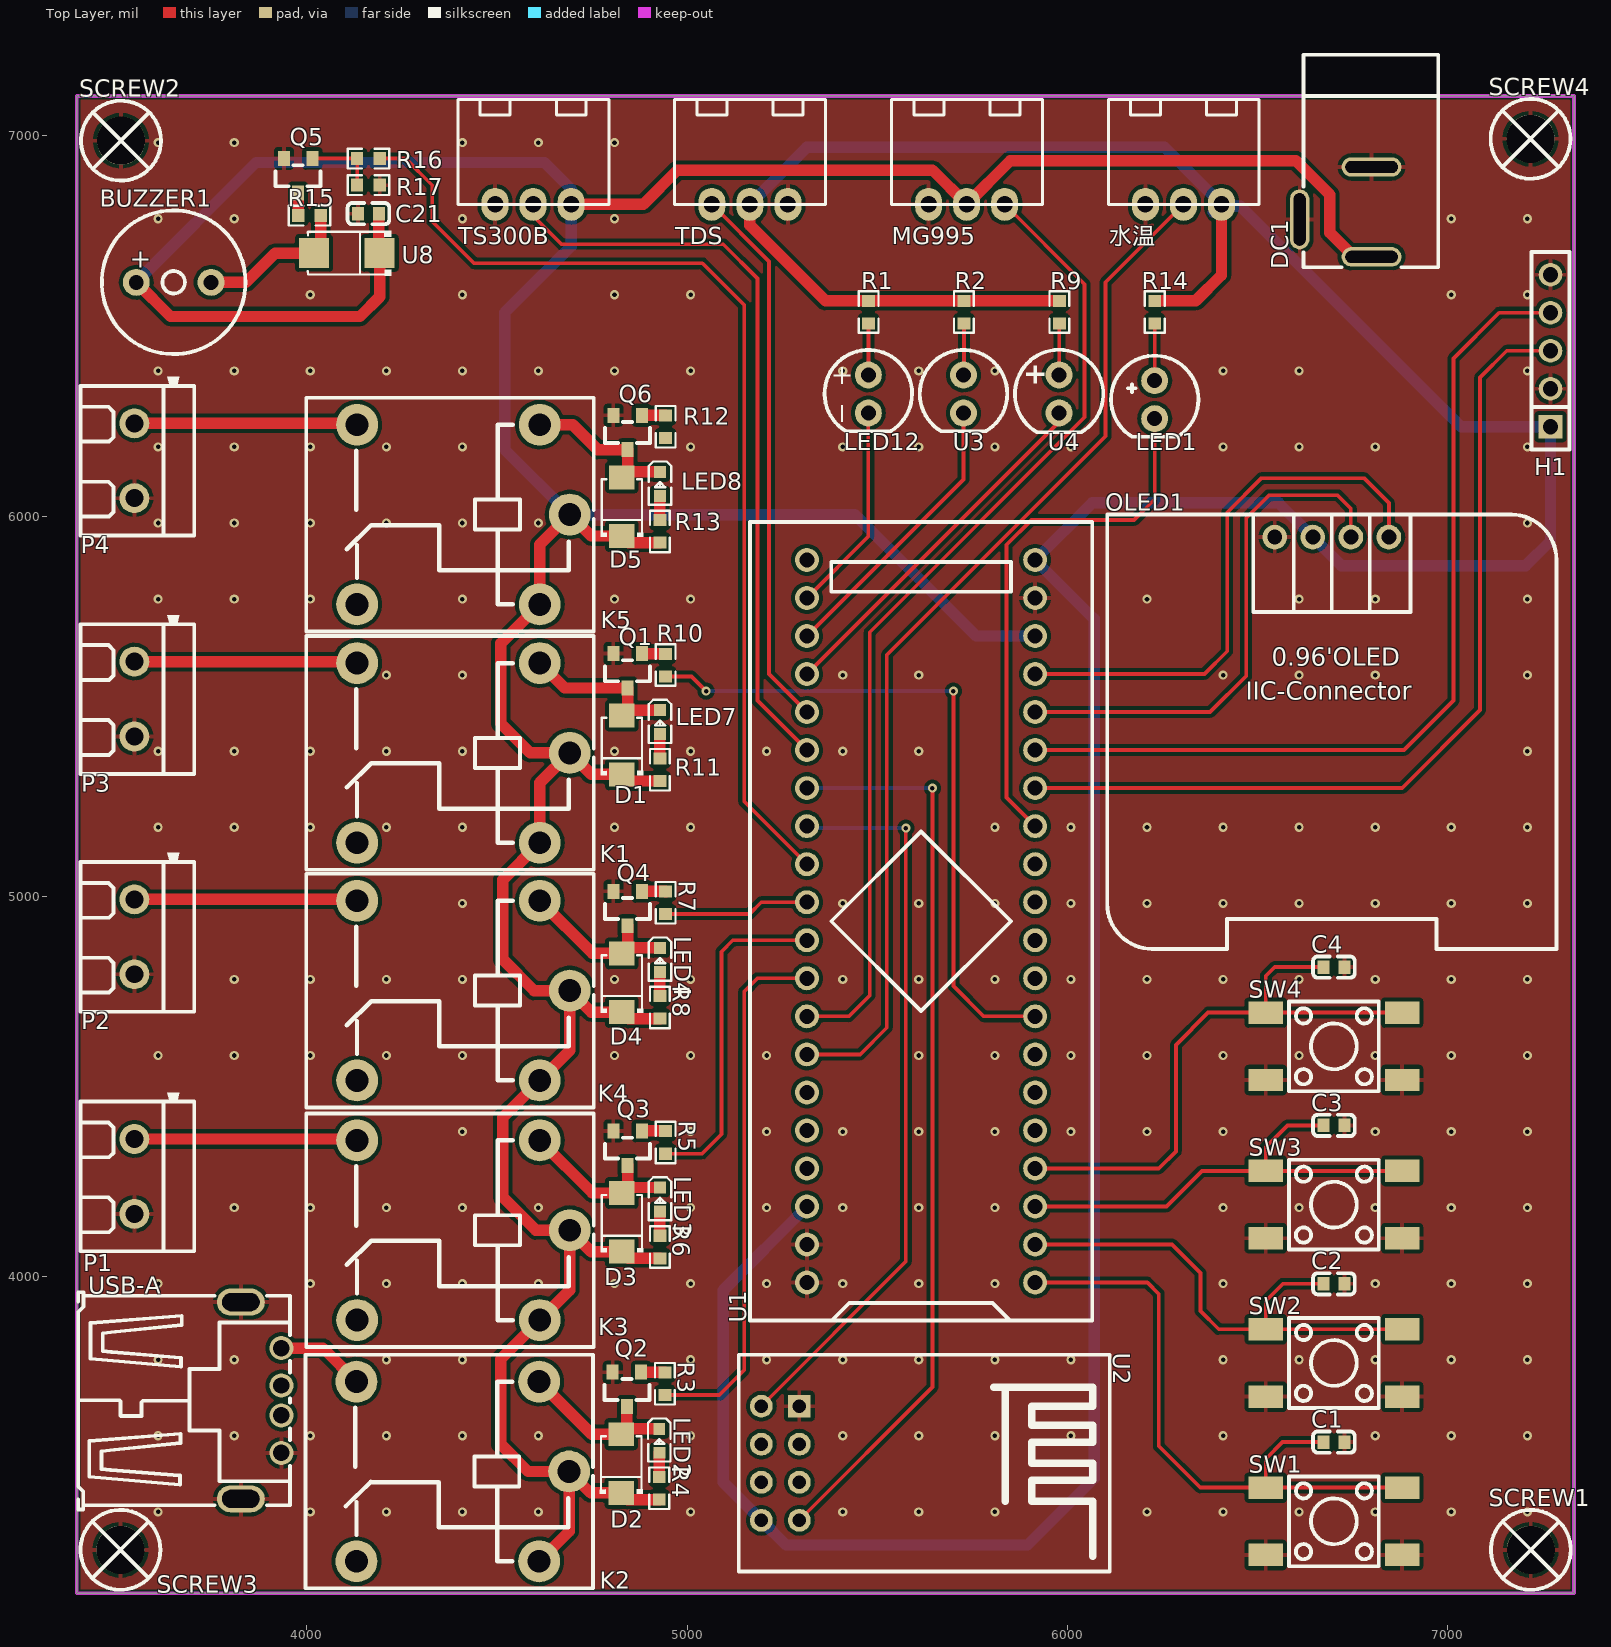
[diagram p0: Top Layer view]
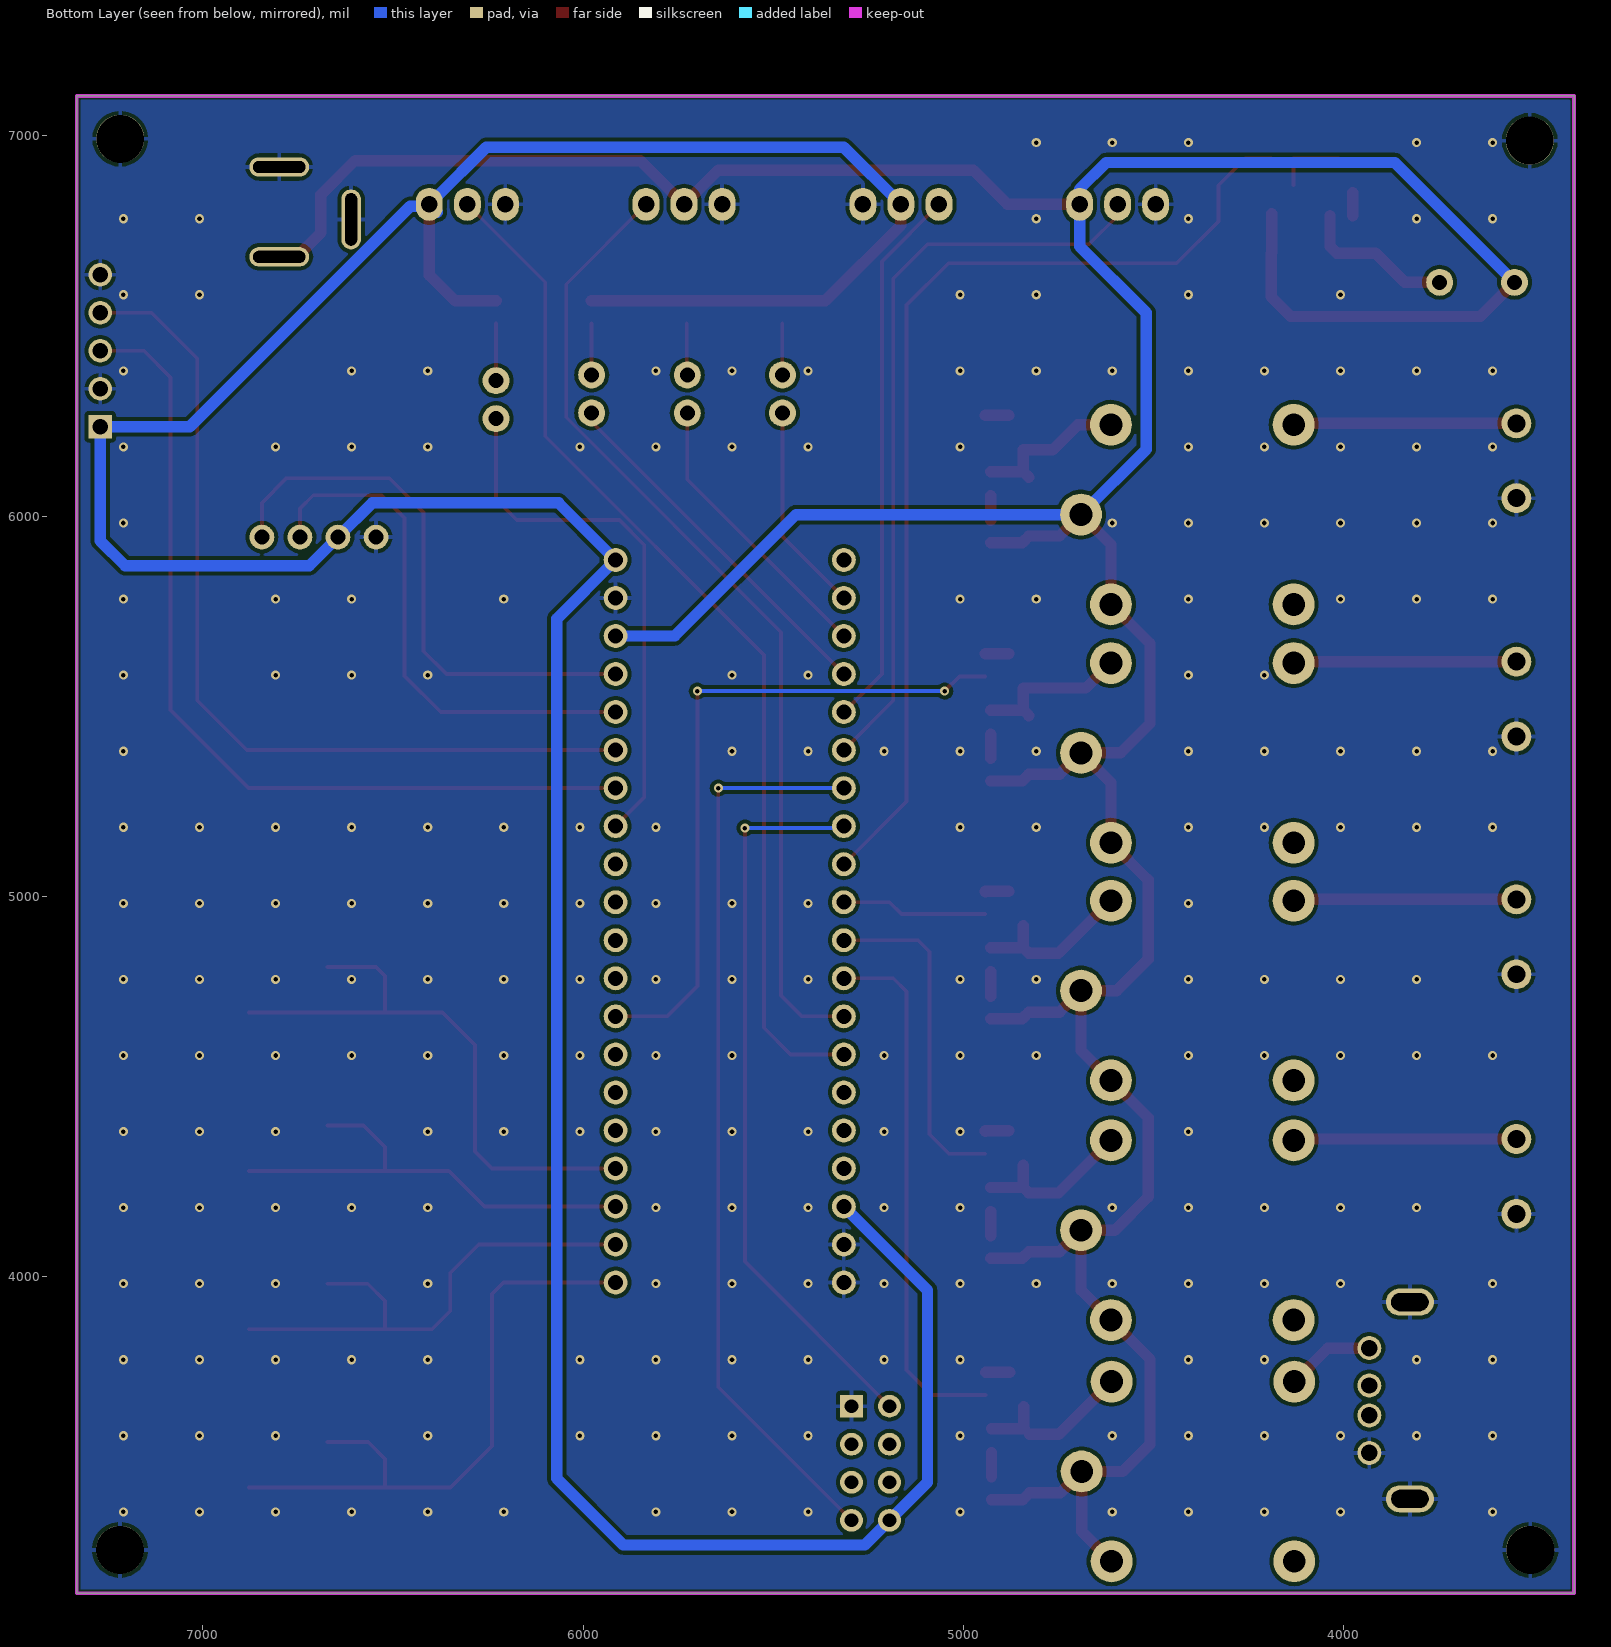
[diagram p1: Bottom Layer view, seen from below]
# Altium PCB MISC51727.pcbdoc
Units mil, origin at the board's own origin, x right, y up, seen from the top; angles counter-clockwise.
Board outline 3937.01 x 3937.01 mil, 2 copper layers (Top Layer, Bottom Layer), stack 62.206 mil thick; 71 components, 56 nets, 225 pads, 231 vias.

## Layer stack, top to bottom
Top Solder Mask Layer: solder mask 0.394, Dk 3.3
Top Layer: signal copper 1.379
Dielectric1: surface 59.449, FR4, Dk 4.5
Bottom Layer: signal copper 1.378
Bottom Solder Mask Layer: solder mask 0.394, Dk 3.3

## Board outline
3395,7105 3395,3167.99 7332.01,3167.99 7332.01,7105

## Design rules (kind name [scope] priority, off if disabled: settings)
BoardOutlineClearance copperThickness2oz_1 [All] p2 off: genericclearance=7.99 ignorepadtopadclearanceinfootprint=FALSE except(0: Arc-SplitContinuation Track-SplitContinuation SMDPad-SplitContinuation THPad-SplitContinuation Via-SplitContinuation Fill-SplitContinuation Region-SplitContinuation Poly-SplitContinuation Text-SplitContinuation Hole-SplitContinuation; 5.98: Arc-CutoutEdge SMDPad-CutoutEdge THPad-CutoutEdge Via-CutoutEdge Fill-CutoutEdge Region-CutoutEdge Text-CutoutEdge; 6.93: Hole-OutlineEdge Hole-CutoutEdge; 10: Poly-OutlineEdge Poly-CutoutEdge; 11.81: Arc-OutlineEdge Track-OutlineEdge SMDPad-OutlineEdge THPad-OutlineEdge Via-OutlineEdge Fill-OutlineEdge Region-OutlineEdge Text-OutlineEdge Track-CutoutEdge)
BoardOutlineClearance copperThickness1oz_1 [All] p4: genericclearance=4.02 ignorepadtopadclearanceinfootprint=FALSE except(0: Arc-SplitContinuation Track-SplitContinuation SMDPad-SplitContinuation THPad-SplitContinuation Via-SplitContinuation Fill-SplitContinuation Region-SplitContinuation Poly-SplitContinuation Text-SplitContinuation Hole-SplitContinuation; 6: SMDPad-CutoutEdge THPad-CutoutEdge Via-CutoutEdge Fill-CutoutEdge Region-CutoutEdge Text-CutoutEdge; 6.93: Hole-OutlineEdge Hole-CutoutEdge; 10: Poly-OutlineEdge Poly-CutoutEdge; 11.8: Arc-OutlineEdge Track-OutlineEdge SMDPad-OutlineEdge THPad-OutlineEdge Via-OutlineEdge Fill-OutlineEdge Region-OutlineEdge Text-OutlineEdge; 11.81: Arc-CutoutEdge Track-CutoutEdge)
Clearance copperThickness2oz [All] p1 off: gap=7.99 ignorepadtopadclearanceinfootprint=FALSE except(5.98: SMDPad-Track SMDPad-SMDPad THPad-Track SMDPad-THPad THPad-THPad Track-Via SMDPad-Via THPad-Via Via-Via Fill-Track Region-Track Fill-SMDPad Region-SMDPad Fill-THPad Region-THPad Fill-Via Region-Via Fill-Fill Fill-Region Region-Region Arc-Track Arc-SMDPad Arc-THPad Arc-Via Fill-Arc Region-Arc Arc-Arc Text-Track SMDPad-Text Text-THPad Text-Via Fill-Text Region-Text Arc-Text Text-Text; 6.93: Hole-Track Hole-SMDPad Hole-THPad Hole-Via Fill-Hole Region-Hole Hole-Arc Hole-Text; 10: Poly-Track Poly-SMDPad Poly-THPad Poly-Via Poly-Fill Poly-Region Poly-Poly Poly-Arc Poly-Text Poly-Hole)
Clearance copperThickness1oz [All] p3: gap=4.02 ignorepadtopadclearanceinfootprint=FALSE except(5.98: SMDPad-Track SMDPad-SMDPad THPad-Track SMDPad-THPad THPad-THPad Track-Via SMDPad-Via THPad-Via Via-Via Fill-Track Region-Track Fill-SMDPad Region-SMDPad Fill-THPad Region-THPad Fill-Via Region-Via Fill-Fill Fill-Region Region-Region; 6: Arc-Track Arc-SMDPad Arc-THPad Arc-Via Fill-Arc Region-Arc Arc-Arc Text-Track SMDPad-Text Text-THPad Text-Via Fill-Text Region-Text Arc-Text Text-Text; 6.93: Hole-Track Hole-SMDPad Hole-THPad Hole-Via Fill-Hole Region-Hole Hole-Arc Hole-Text; 10: Poly-Track Poly-SMDPad Poly-THPad Poly-Via Poly-Fill Poly-Region Poly-Poly Poly-Arc Poly-Text Poly-Hole)
Creepage creepage [All] p1: checkdistance=0 ignoreinternallayers=TRUE applytopolygonpour=TRUE
DiffPairsRouting differentialPair [All] p1: maxlimit=6 minlimit=6 mostfreqgap=6 toplayer_minwidth=5 toplayer_prefwidth=10 toplayer_maxwidth=100 toplayer_mingap=6 toplayer_prefgap=6 toplayer_maxgap=6 bottomlayer_minwidth=5 bottomlayer_prefwidth=10 bottomlayer_maxwidth=100 bottomlayer_mingap=6 bottomlayer_prefgap=6 bottomlayer_maxgap=6 maxuncoupledlength=10
HoleToHoleClearance otherClearance [All] p1: gap=11.81 allowstackedmicrovias=TRUE
Length netLength [All] p1: minlimit=0 maxlimit=0
MatchedLengths netLengthTolerance [All] p1: tolerance=1000
PasteMaskExpansion pasteMaskExpansion [All] p1: expansion=0
PlaneConnect innerPlane [All] p1: planeconnectstyle=Relief reliefexpansion=20 reliefentries=4 reliefconductorwidth=10 reliefairgap=10
PolygonConnect copperRegion [(InNet('GND'))] p1: connectstyle=Relief reliefconductorwidth=10 reliefentries=4 polygonreliefangle="90 Angle" airgapwidth=10 via.connectstyle=Relief via.reliefconductorwidth=10 via.reliefentries=4 via.polygonreliefangle="90 Angle" via.airgapwidth=10
RoutingVias viaSize [All] p1: holewidth=12.01 width=24.02 viastyle="Through Hole" minholewidth=11.81 minwidth=19.68 maxholewidth=248.03 maxwidth=393.7
SolderMaskExpansion solderMaskExpansion [IsVia] p1: expansion=-1000 istentingtop=TRUE
SolderMaskExpansion solderMaskExpansion [All] p2: expansion=2 istentingtop=FALSE
Width copperThickness2oz_2 [All] p1 off: maxlimit=100 minlimit=8 preferedwidth=10
Width copperThickness1oz_2 [All] p2: maxlimit=100 minlimit=5 preferedwidth=10

## Components (designator, comment, footprint, x,y, rotation, side; value= is the part's Value field where it differs from the comment)
BUZZER1 "3kHz" BUZ-TH_BD9.6-P5.00-D0.7-FD 3650,6615 r0 top
C1 "100nF" C0603 6700.55,3565.55 r0 top
C2 "100nF" C0603 6700.55,3981.81 r0 top
C3 "100nF" C0603 6700.55,4398.07 r0 top
C4 "100nF" C0603 6700.55,4814.33 r0 top
C21 "100nF" C0603 4162.11,6795.28 r0 top
D1 "M7F" SMAF_L3.5-W2.6-LS4.7-RD 4828.38,5398.43 r90 top
D2 "M7F" SMAF_L3.5-W2.6-LS4.7-RD 4826.72,3509.06 r90 top
D3 "M7F" SMAF_L3.5-W2.6-LS4.7-RD 4828.38,4143.43 r90 top
D4 "M7F" SMAF_L3.5-W2.6-LS4.7-RD 4828.38,4773.43 r90 top
D5 "M7F" SMAF_L3.5-W2.6-LS4.7-RD 4828.38,6025.08 r90 top
DC1 "" DC-2.0 6810,6805 r90 top
H1 "" HDR-TH_5P-P2.54-V-F 7270,6435 r90 top
K1 "SRD-DC5V-SL-C" RELAY-TH_SRD-DCXXV-SL-C 4411.82,5377.66 r180 top
K2 "SRD-DC5V-SL-C" RELAY-TH_SRD-DCXXV-SL-C 4410.16,3488.29 r180 top
K3 "SRD-DC5V-SL-C" RELAY-TH_SRD-DCXXV-SL-C 4411.82,4122.66 r180 top
K4 "SRD-DC5V-SL-C" RELAY-TH_SRD-DCXXV-SL-C 4411.82,4752.66 r180 top
K5 "SRD-DC5V-SL-C" RELAY-TH_SRD-DCXXV-SL-C 4411.82,6004.31 r180 top
LED1 "blue" LED-TH_BD5.9-P2.54-RD_BLUE 6229.4,6306.44 r90 top
LED2 "MS-PTV1608NWAF-B02" LED0603-RD 4926.72,3569.06 r270 top
LED3 "MS-PTV1608NWAF-B02" LED0603-RD 4928.38,4203.43 r270 top
LED4 "MS-PTV1608NWAF-B02" LED0603-RD 4928.38,4833.43 r270 top
LED7 "MS-PTV1608NWAF-B02" LED0603-RD 4928.38,5458.43 r270 top
LED8 "MS-PTV1608NWAF-B02" LED0603-RD 4928.38,6085.08 r270 top
LED12 "red" LED-TH_BD5.9-P2.54-RD_RED 5476.39,6321.24 r90 top
MG995 "" XH2.54-3P 5735,6820 r0 top
OLED1 "" 0.96OLED_4P 6695,5945 r0 top
P1 "KF301-2P terminal block" CONN-TH_XY301V-A-5.0-2P 3546.72,4264.06 r90 top
P2 "KF301-2P terminal block" CONN-TH_XY301V-A-5.0-2P 3546.72,4894.06 r90 top
P3 "KF301-2P terminal block" CONN-TH_XY301V-A-5.0-2P 3546.72,5519.06 r90 top
P4 "KF301-2P terminal block" CONN-TH_XY301V-A-5.0-2P 3546.72,6145.71 r90 top
Q1 "" S8050_SOT-23 4848.38,5593.43 r90 top
Q2 "" S8050_SOT-23 4846.72,3704.06 r90 top
Q3 "" S8050_SOT-23 4848.38,4338.43 r90 top
Q4 "" S8050_SOT-23 4848.38,4968.43 r90 top
Q5 "" S8050_SOT-23 3982.11,6895.28 r90 top
Q6 "" S8050_SOT-23 4848.38,6220.08 r90 top
R1 "1K" R0603 5477.06,6536.64 r270 top
R2 "1K" R0603 5727.84,6536.64 r270 top
R3 "330" R0603 4941.72,3719.06 r270 top
R4 "1K" R0603 4926.72,3444.06 r270 top
R5 "330" R0603 4943.38,4353.43 r270 top
R6 "1K" R0603 4928.38,4078.43 r270 top
R7 "330" R0603 4943.38,4983.43 r270 top
R8 "1K" R0603 4928.38,4708.43 r270 top
R9 "1K" R0603 5978.62,6536.64 r270 top
R10 "330" R0603 4943.38,5608.43 r270 top
R11 "1K" R0603 4928.38,5333.43 r270 top
R12 "330" R0603 4943.38,6235.08 r270 top
R13 "1K" R0603 4928.38,5960.08 r270 top
R14 "1K" R0603 6229.4,6536.64 r270 top
R15 "0R" R0603 4007.11,6790.28 r0 top
R16 "1K" R0603 4162.11,6940.28 r0 top
R17 "4.7K" R0603 4162.11,6870.28 r0 top
SCREW1 "" M3螺丝 7218.26,3282.26 r0 top
SCREW2 "" M3螺丝 3511.56,6987.26 r0 top
SCREW3 "" M3螺丝 3510,3282.26 r0 top
SCREW4 "" M3螺丝 7217.52,6992.26 r0 top
SW1 "" SW-SMD_4P-L6.0-W6.0-P4.50-LS9.0-2 6700.55,3357.42 r0 top
SW2 "" SW-SMD_4P-L6.0-W6.0-P4.50-LS9.0-2 6700.55,3773.68 r0 top
SW3 "" SW-SMD_4P-L6.0-W6.0-P4.50-LS9.0-2 6700.55,4189.94 r0 top
SW4 "" SW-SMD_4P-L6.0-W6.0-P4.50-LS9.0-2 6700.55,4606.2 r0 top
TDS "" XH2.54-3P 5165,6820 r0 top
TS300B "" XH2.54-3P 4595,6820 r0 top
U1 "LCKFB-DKX-STM32F103C8T6" CONN-TH_L53.3-W22.9_STM32F103C8T6-CARD 5615,4935 r90 top
U2 "ESP8266-01S" WIFIM-TH_ESP8266-01S 5245,3510 r270 top
U3 "green" LED-TH_BD5.9-P2.54-RD_GREEN 5726.63,6321.14 r90 top
U4 "yellow" LED-TH_BD5.9-P2.54-RD_YELLOW 5977.95,6321.4 r90 top
U8 "SS24-MS" SMA_L4.3-W2.6-LS5.1-RD 4105.13,6691.58 r180 top
USB-A "USB-AF" USB-A-TH_USB-302-T 3880,3675 r270 top
水温 "" XH2.54-3P 6305,6820 r0 top

## Footprints (in the part's own frame and the unit in brackets; to place one, negate y for a bottom-side part, rotate by r counter-clockwise, add the part's x,y. Pads: shape width x height; smd on the part's side, far side on the other; paste and mask are expansions set on the pad)
0.96OLED_4P [mm]
  round 1.65 hole 1 copper offset 0,0: 1(-3.81,-0.001) 2(-1.27,0.002) 3(1.27,0.002) 4(3.81,0.002)
  silkscreen extent -15,-27.5 15,1.5
BUZ-TH_BD9.6-P5.00-D0.7-FD [mm]
  round 1.8 hole 1: 1(-2.5,0) 2(2.5,0)
  silkscreen extent -4.8,-4.8 4.8,4.8
C0603 [mm]
  rect 0.8x0.9 smd: 1(-0.7,0) 2(0.7,0)
  silkscreen extent -1.39,-0.71 1.39,0.71
CONN-TH_L53.3-W22.9_STM32F103C8T6-CARD [mm]
  round 1.6 hole 1: 1(-24.13,-7.62) 2(-21.59,-7.62) 3(-19.05,-7.62) 4(-16.51,-7.62) 5(-13.97,-7.62) 6(-11.43,-7.62) 7(-8.89,-7.62) 8(-6.35,-7.62) 9(-3.81,-7.62) 10(-1.27,-7.62) 11(1.27,-7.62) 12(3.81,-7.62) 13(6.35,-7.62) 14(8.89,-7.62) 15(11.43,-7.62) 16(13.97,-7.62) 17(16.51,-7.62) 18(19.05,-7.62) 19(21.59,-7.62) 20(24.13,-7.62) 21(24.13,7.62) 22(21.59,7.62) 23(19.05,7.62) 24(16.51,7.62) 25(13.97,7.62) 26(11.43,7.62) 27(8.89,7.62) 28(6.35,7.62) 29(3.81,7.62) 30(1.27,7.62) 31(-1.27,7.62) 32(-3.81,7.62) 33(-6.35,7.62) 34(-8.89,7.62) 35(-11.43,7.62) 36(-13.97,7.62) 37(-16.51,7.62) 38(-19.05,7.62) 39(-21.59,7.62) 40(-24.13,7.62)
  silkscreen extent -26.67,-11.43 26.67,11.43
CONN-TH_XY301V-A-5.0-2P [mm]
  round 2 hole 1.2: 1(-2.5,0) 2(2.5,0)
  silkscreen extent -5,-4 5.6,3.6
DC-2.0 [mil]
  oval 157.5x51.2 hole 31.5 slot 137.8 at 0 deg paste+0 mask+2: 2(-24.7,199.5)
  oval 51.2x157.5 hole 31.5 slot 137.8 at 90 deg paste+0 mask+2: 3(113.1,10.5) 4(-123.1,10.5)
  silkscreen extent -151,-165 408,190
HDR-TH_5P-P2.54-V-F [mil]
  rect 62x62 hole 40.16: 1(-200,0)
  round 62 hole 40.16: 2(-100,0) 3(0,0) 4(100,0) 5(200,0)
  silkscreen extent -260,-50 260,50
LED0603-RD [mm]
  rect 0.8x0.8 smd: 1(-0.799,0) 2(0.799,0)
  silkscreen extent -1.49,-0.75 1.39,0.76
LED-TH_BD5.9-P2.54-RD_BLUE [mm]
  round 1.8 hole 1 paste+0 mask+0.05: 1(-1.27,0) 2(1.27,0)
  silkscreen extent -2.49,-2.92 2.93,2.92
LED-TH_BD5.9-P2.54-RD_GREEN [mm]
  round 1.8 hole 1 paste+0 mask+0.05: 1(-1.27,0) 2(1.27,0)
  silkscreen extent -2.49,-2.92 2.94,2.92
LED-TH_BD5.9-P2.54-RD_RED [mm]
  round 1.8 hole 1 paste+0 mask+0.05: 1(-1.27,0) 2(1.27,0)
  silkscreen extent -2.49,-2.92 2.94,2.92
LED-TH_BD5.9-P2.54-RD_YELLOW [mm]
  round 1.8 hole 1 paste+0 mask+0.05: 1(-1.27,0) 2(1.27,0)
  silkscreen extent -2.55,-2.95 2.95,2.95
M3螺丝 [mil]
  round 126 hole 126 paste+0 mask+4: 1(0,0)
  silkscreen extent -105,-105 105,105
R0603 [mil]
  rect 31.75x34.02 smd paste-3937.01 mask+2: 1(-29.66,0) 2(29.66,0)
  silkscreen extent -55,-26 55,26
RELAY-TH_SRD-DCXXV-SL-C [mil]
  round 110 hole 60: 1(-200.79,-236.22) 2(279.53,-236.2) 3(279.53,236.2) 4(-200.79,236.22) 5(-279.53,0)
  silkscreen extent -342,-307 413,307
S8050_SOT-23 [mm]
  rect 1x0.8 smd paste+0 mask+0.051: 1(1.15,-0.823) 2(1.15,1.077) 3(-1.15,0.127)
  silkscreen extent -0.7,-1.37 0.7,1.63
SMA_L4.3-W2.6-LS5.1-RD [mm]
  rect 2x2 smd: 1(-2.2,0) 2(2.2,0)
  silkscreen extent -2.98,-1.5 2.6,1.5
SMAF_L3.5-W2.6-LS4.7-RD [mm]
  rect 1.6x1.7 smd: 1(-1.96,0) 2(1.96,0)
  silkscreen extent -2.01,-1.43 1.83,1.42
SW-SMD_4P-L6.0-W6.0-P4.50-LS9.0-2 [mm]
  rect 2.3x1.5 smd: 1(-4.55,2.25) 2(4.55,2.25) 3(-4.55,-2.25) 4(4.55,-2.25)
  silkscreen extent -3,-3 3,3
USB-A-TH_USB-302-T [mm]
  round 1.6 hole 1.1: 1(-3.5,1.355) 2(-1,1.355) 3(1,1.355) 4(3.5,1.355)
  oval 1.8x3.2 hole 1.2 slot 2.5 at 90 deg copper offset -0.001,-0.001: 5(-6.569,-1.354)
  oval 1.8x3.2 hole 1.2 slot 2.5 at 90 deg copper offset 0.001,0.001: 6(6.569,-1.356)
  silkscreen extent -7.23,-12.21 7.28,1.92
WIFIM-TH_ESP8266-01S [mil]
  rect 60x60 hole 36 paste+0 mask+1.97: 1(-150,50)
  round 60 hole 36 paste+0 mask+1.97: 2(-50,50) 3(50,50) 4(150,50) 5(-150,-50) 6(-50,-50) 7(50,-50) 8(150,-50)
  silkscreen extent -285,-109 285,866
XH2.54-3P [mm]
  oval 1.8x2.2 hole 1.1 paste+0 mask+0.102: 1(-2.54,0) 2(0,0) 3(2.54,0)
  silkscreen extent -5.02,0 5.05,7

## Via types
v1: diameter 24.02, hole 12, Top Layer to Bottom Layer, 231 vias

## Nets (pads, with @x,y where several pads share a name; then routed paths per layer and width w, separated by ;. In a path a pad name is that pad's centre, name@x,y a point inside that pad or via, vN(x,y) a via of type N, cw(c..) or ccw(c..) an arc to the next point about the centre after c; other vN are vias at no path point)
$1N2314: Q2.1 R3.1 | length 62.9
  Top Layer w30: Q2.1 4941.11,3749.34 R3.1
$1N2315: D2.2 K2.1 LED2.1 Q2.3 | length 417.3
  Top Layer w30: K2.1 4749.24,3586.23 D2.2 ; Q2.3 4841.72,3601.23 4841.03,3600.54 LED2.1
$1N2316: LED2.2 R4.1 | length 63.9
  Top Layer w30: R4.1 LED2.2
$1N2322: D3.2 K3.1 LED3.1 Q3.3 | length 437.5
  Top Layer w30: K3.1 4750.89,4220.6 D3.2 D3.2@4842.69,4234.91 ; Q3.3 4843.38,4235.6 D3.2@4842.69,4234.91 ; LED3.1 D3.2@4842.69,4234.91
$1N2323: LED3.2 R6.1 | length 63.9
  Top Layer w30: R6.1 LED3.2
$1N2328: Q3.1 R5.1 | length 62.9
  Top Layer w30: Q3.1 4942.76,4383.71 R5.1
$1N2330: Q4.1 R7.1 | length 62.9
  Top Layer w30: Q4.1 4942.76,5013.71 R7.1
$1N2331: D4.2 K4.1 LED4.1 Q4.3 | length 437.5
  Top Layer w30: K4.1 4750.89,4850.6 D4.2 D4.2@4842.69,4864.91 ; Q4.3 4843.38,4865.6 D4.2@4842.69,4864.91 ; LED4.1 D4.2@4842.69,4864.91
$1N2332: LED4.2 R8.1 | length 63.9
  Top Layer w30: R8.1 LED4.2
$1N2355: BUZZER1.2 R15.2 U8.2 | length 408.1
  Top Layer w30: BUZZER1.2 3840,6615 3916.58,6691.58 U8.2 4036.77,6709.84 R15.2
$1N2356: Q5.1 R16.1 R17.1 | length 188.1
  Top Layer w10: Q5.1 4014.79,6940.28 R16.1 R17.1
$1N2361: Q5.3 R15.1 | length 59.9
  Top Layer w30: Q5.3 3977.45,6849.67 R15.1
$1N3430: K2.2 USB-A.1 | length 233.9
  Top Layer w30: USB-A.1 4042.34,3812.79 K2.2
$1N8411: K4.2 P2.2 | length 587.1
  Top Layer w30: P2.2 4128.66,4992.49 K4.2
$1N8431: K3.2 P1.2 | length 587.1
  Top Layer w30: P1.2 4128.66,4362.49 K3.2
$1N8484: R9.2 U4.2 | length 135.9
  Top Layer w10: U4.2 5978.62,6372.07 R9.2
$1N8493: K1.2 P3.2 | length 587.1
  Top Layer w30: P3.2 4128.66,5617.49 K1.2
$1N8495: Q1.1 R10.1 | length 62.9
  Top Layer w30: Q1.1 4942.76,5638.71 R10.1
$1N8497: LED7.2 R11.1 | length 63.9
  Top Layer w30: R11.1 LED7.2
$1N8498: D1.2 K1.1 LED7.1 Q1.3 | length 422.4
  Top Layer w30: K1.1 4678.33,5548.16 Q1.3 4843.38,5490.6 D1.2@4842.69,5489.91 ; D1.2 D1.2@4842.69,5489.91 ; LED7.1 D1.2@4842.69,5489.91
$1N8520: K5.2 P4.2 | length 587.1
  Top Layer w30: P4.2 4128.66,6244.13 K5.2
$1N8522: Q6.1 R12.1 | length 62.9
  Top Layer w30: Q6.1 4942.76,6265.35 R12.1
$1N8524: LED8.2 R13.1 | length 63.9
  Top Layer w30: R13.1 LED8.2
$1N8525: D5.2 K5.1 LED8.1 Q6.3 | length 422.4
  Top Layer w30: K5.1 4699.47,6240.53 4765.2,6174.8 Q6.3 4843.38,6117.24 D5.2@4842.69,6116.55 ; D5.2 D5.2@4842.69,6116.55 ; LED8.1 D5.2@4842.69,6116.55
$1N8526: LED12.2 R1.2 | length 136
  Top Layer w10: LED12.2 5477.06,6371.91 R1.2
$1N8527: R2.2 U3.2 | length 136.3
  Top Layer w10: U3.2 5727.84,6372.36 R2.2
$1N8528: LED1.2 R14.2 | length 150.5
  Top Layer w10: LED1.2 R14.2
+5V: BUZZER1.1 C21.2 D1.1 D2.1 D3.1 D4.1 D5.1 DC1.4 K1.4 K1.5 K2.4 K2.5 K3.4 K3.5 K4.4 K4.5 K5.4 K5.5 MG995.2 R4.2 R6.2 R8.2 R11.2 R13.2 TS300B.3 U1.18 U8.1 | length 11912.7
  Top Layer w30: BUZZER1.1 3641.57,6525 4140,6525 4191.74,6576.74 U8.1 4189.67,6693.66 C21.2 ; K2.4 4689.69,3330.81 K2.5 ; TS300B.3 4885,6820 4975,6910 5645,6910 MG995.2 5849.99,6935 6600,6935 6690,6845 6690,6745 6753.1,6681.9 DC1.4 ; R4.2 4844.22,3414.4 D2.1 4746.09,3431.9 K2.5 ; R6.2 4845.87,4048.77 D3.1 4747.74,4066.27 K3.5 ; R8.2 4845.87,4678.77 D4.1 4747.74,4696.27 K4.5 ; R11.2 4845.87,5303.77 D1.1 4747.74,5321.27 K1.5 ; R13.2 4845.87,5930.42 D5.1 4747.74,5947.91 K5.5 4612.61,5925.57 K5.4 4510,5665.48 4510,5455 4587.34,5377.66 K1.5 ; K2.5 4581.71,3488.29 4510,3560 4510,3783.83 K3.4 4691.35,3965.18 K3.5 ; K3.5 4602.34,4122.66 4515,4210 4515,4418.83 K4.4 4691.35,4595.18 K4.5 ; K4.5 4597.34,4752.66 4515,4835 4515,5043.83 K1.4 4612.61,5298.92 K1.5
  Bottom Layer w30: BUZZER1.1 3866.57,6930 4625,6930 4695,6860 TS300B.3 4695,6710 4520,6535 4520,6175.66 K5.5 5440.69,6004.31 5760,5685 U1.18
GND: C1.2 C2.2 C3.2 C4.2 C21.1 DC1.2 DC1.3 H1.2 H1.5 MG995.1 OLED1.1 P1.1 P2.1 P3.1 P4.1 Q1.2 Q2.2 Q3.2 Q4.2 Q5.2 Q6.2 R17.2 SCREW1.1 SCREW2.1 SCREW3.1 SCREW4.1 SW1.3 SW1.4 SW2.3 SW2.4 SW3.3 SW3.4 SW4.3 SW4.4 TDS.3 TS300B.1 U1.19 U1.39 U1.40 U2.1 USB-A.4 USB-A.5 USB-A.6 水温.1
  other v1: 3609.1,3382.09 4009.1,3382.09 4209.1,3382.09 4409.1,3382.09 4609.1,3382.09 5009.1,3382.09 5409.1,3382.09 5609.1,3382.09 5809.1,3382.09 6209.1,3382.09 6409.1,3382.09 6609.1,3382.09 6809.1,3382.09 7009.1,3382.09 7209.1,3382.09 3609.1,3582.09 3809.1,3582.09 4009.1,3582.09 4209.1,3582.09 4409.1,3582.09 4609.1,3582.09 5009.1,3582.09 5409.1,3582.09 5609.1,3582.09 5809.1,3582.09 6009.1,3582.09 6409.1,3582.09 6809.1,3582.09 7009.1,3582.09 7209.1,3582.09 3609.1,3782.09 3809.1,3782.09 4209.1,3782.09 4409.1,3782.09 5009.1,3782.09 5209.1,3782.09 5409.1,3782.09 5609.1,3782.09 5809.1,3782.09 6009.1,3782.09 6409.1,3782.09 6609.1,3782.09 6809.1,3782.09 7009.1,3782.09 7209.1,3782.09 3609.1,3982.09 4009.1,3982.09 4209.1,3982.09 4409.1,3982.09 4609.1,3982.09 4809.1,3982.09 5009.1,3982.09 5209.1,3982.09 5409.1,3982.09 5609.1,3982.09 5809.1,3982.09 6409.1,3982.09 6809.1,3982.09 7009.1,3982.09 7209.1,3982.09 3809.1,4182.09 4009.1,4182.09 4209.1,4182.09 4409.1,4182.09 4609.1,4182.09 5009.1,4182.09 5209.1,4182.09 5409.1,4182.09 5609.1,4182.09 5809.1,4182.09 6409.1,4182.09 6609.1,4182.09 6809.1,4182.09 7009.1,4182.09 7209.1,4182.09 4409.1,4382.09 5009.1,4382.09 5209.1,4382.09 5409.1,4382.09 5609.1,4382.09 5809.1,4382.09 6009.1,4382.09 6209.1,4382.09 6409.1,4382.09 6809.1,4382.09 7009.1,4382.09 7209.1,4382.09 3609.1,4582.09 3809.1,4582.09 4009.1,4582.09 4209.1,4582.09 4409.1,4582.09 4809.1,4582.09 5009.1,4582.09 5209.1,4582.09 5609.1,4582.09 5809.1,4582.09 6009.1,4582.09 6209.1,4582.09 6409.1,4582.09 6609.1,4582.09 6809.1,4582.09 7009.1,4582.09 7209.1,4582.09 3809.1,4782.09 4009.1,4782.09 4209.1,4782.09 4409.1,4782.09 4809.1,4782.09 5009.1,4782.09 5409.1,4782.09 5609.1,4782.09 5809.1,4782.09 6009.1,4782.09 6209.1,4782.09 6409.1,4782.09 6609.1,4782.09 6809.1,4782.09 7009.1,4782.09 7209.1,4782.09 4409.1,4982.09 5409.1,4982.09 5609.1,4982.09 5809.1,4982.09 6009.1,4982.09 6209.1,4982.09 6409.1,4982.09 6609.1,4982.09 6809.1,4982.09 7009.1,4982.09 7209.1,4982.09 3609.1,5182.09 3809.1,5182.09 4009.1,5182.09 4209.1,5182.09 4409.1,5182.09 4809.1,5182.09 5009.1,5182.09 5809.1,5182.09 6009.1,5182.09 6209.1,5182.09 6409.1,5182.09 6609.1,5182.09 6809.1,5182.09 7009.1,5182.09 7209.1,5182.09 3609.1,5382.09 3809.1,5382.09 4009.1,5382.09 4209.1,5382.09 4409.1,5382.09 4809.1,5382.09 5009.1,5382.09 5209.1,5382.09 5409.1,5382.09 5609.1,5382.09 7209.1,5382.09 4209.1,5582.09 4409.1,5582.09 5409.1,5582.09 5609.1,5582.09 6409.1,5582.09 6609.1,5582.09 6809.1,5582.09 7209.1,5582.09 3609.1,5782.09 3809.1,5782.09 4009.1,5782.09 4409.1,5782.09 4809.1,5782.09 5009.1,5782.09 6209.1,5782.09 6609.1,5782.09 6809.1,5782.09 7209.1,5782.09 3609.1,5982.09 3809.1,5982.09 4009.1,5982.09 4209.1,5982.09 4409.1,5982.09 4609.1,5982.09 7209.1,5982.09 3609.1,6182.09 3809.1,6182.09 4009.1,6182.09 4209.1,6182.09 4409.1,6182.09 5009.1,6182.09 5409.1,6182.09 5609.1,6182.09 5809.1,6182.09 6009.1,6182.09 6409.1,6182.09 6609.1,6182.09 6809.1,6182.09 7209.1,6182.09 3609.1,6382.09 3809.1,6382.09 4009.1,6382.09 4209.1,6382.09 4409.1,6382.09 4609.1,6382.09 4809.1,6382.09 5009.1,6382.09 5409.1,6382.09 5609.1,6382.09 5809.1,6382.09 6409.1,6382.09 6609.1,6382.09 7209.1,6382.09 4009.1,6582.09 4409.1,6582.09 4809.1,6582.09 5009.1,6582.09 7009.1,6582.09 7209.1,6582.09 3609.1,6782.09 3809.1,6782.09 4409.1,6782.09 4809.1,6782.09 7009.1,6782.09 7209.1,6782.09 3609.1,6982.09 3809.1,6982.09 4409.1,6982.09 4609.1,6982.09 4809.1,6982.09
PA0: TDS.1 U1.25 | length 1438.6
  Top Layer w10: TDS.1 5215,6670 5215,5585 U1.25
PA1: TS300B.2 U1.26 | length 1982.2
  Top Layer w10: TS300B.2 4595,6790 4670,6715 5095,6715 5185,6625 5185,5515 U1.26
PA2: U1.27 U2.4 | length 2400
  Top Layer w10: U2.4 5645,3710 v1(5645,5285)
  Bottom Layer w10: U1.27 v1(5645,5285)
PA3: U1.28 U2.5 | length 1939.5
  Top Layer w10: U2.5 5575,4040 v1(5575,5180)
  Bottom Layer w10: U1.28 5320,5180 v1(5575,5180)
PA4: R16.2 U1.29 | length 2711.8
  Top Layer w10: R16.2 4259.72,6940.28 4330,6870 4330,6775 4440,6665 5040,6665 5150,6555 5150,5250 U1.29
PA5: R7.2 U1.30 | length 384.6
  Top Layer w10: R7.2 5163.77,4953.77 5195,4985 U1.30
PA6: R5.2 U1.31 | length 885.3
  Top Layer w10: R5.2 5038.77,4323.77 5090,4375 5090,4855 5120,4885 U1.31
PA7: R3.2 U1.32 | length 1409.9
  Top Layer w10: R3.2 5084.4,3689.4 5150,3755 5150,4750 5185,4785 U1.32
PA11: R10.2 U1.8 | length 1795.8
  Top Layer w10: R10.2 5011.23,5578.77 v1(5050,5540) ; v1(5700,5540) 5700,4765 5780,4685 U1.8
  Bottom Layer w10: v1(5050,5540) v1(5700,5540)
PA12: R12.2
PB0: MG995.3 U1.33 | length 2588.8
  Top Layer w10: U1.33 5425,4685 5480,4740 5480,5695 6045,6260 6045,6610 MG995.3
PB1: U1.34 水温.2 | length 2727.1
  Top Layer w10: U1.34 5455,4585 5525,4655 5525,5635 6100,6210 6100,6615.01 水温.2
PB5: LED1.1 U1.13 | length 1422
  Top Layer w10: U1.13 5840,5260 5840,5925 5905,5990 6175,5990 6229.4,6044.4 LED1.1
PB6: H1.3 U1.14 | length 2343.9
  Top Layer w10: U1.14 6880,5285 7085,5490 7085,6365 7155,6435 H1.3
PB7: H1.4 U1.15 | length 2358.6
  Top Layer w10: U1.15 6885,5385 7015,5515 7015,6415 7135,6535 H1.4
PB8: OLED1.3 U1.16 | length 1398.7
  Top Layer w10: U1.16 6375,5485 6470,5580 6470,5995 6530,6055 6710,6055 6745,6020 OLED1.3@6745,5945.05
PB9: OLED1.4 U1.17 | length 1474
  Top Layer w10: U1.17 6360,5585 6420,5645 6420,6010 6510,6100 6780,6100 6845,6035 OLED1.4@6845,5945.05
PB12: C1.1 SW1.1 SW1.2 U1.1 | length 1667.5
  Top Layer w10: U1.1 6210,3985 6240,3955 6240,3555 6349,3446 SW1.1 ; C1.1 6565.55,3565.55 6521.42,3521.42 SW1.1 ; SW1.2 SW1.1
PB13: C2.1 SW2.1 SW2.2 U1.2 | length 1360
  Top Layer w10: U1.2 6275,4085 6350,4010 6350,3910 6397.74,3862.26 SW2.1 ; C2.1 6566.81,3981.81 6521.42,3936.42 SW2.1 ; SW2.2 SW2.1
PB14: C3.1 SW3.1 SW3.2 U1.3 | length 1241.3
  Top Layer w10: U1.3 6260,4185 6353.52,4278.52 SW3.1 ; C3.1 6578.07,4398.07 6521.42,4341.42 SW3.1 ; SW3.2 SW3.1
PB15: C4.1 SW4.1 SW4.2 U1.4 | length 1556.7
  Top Layer w10: U1.4 6240,4285 6285,4330 6285,4610 6369.78,4694.78 SW4.1 ; C4.1 6672.33,4815 6545,4815 6521.42,4791.42 SW4.1 ; SW4.2 SW4.1
PC13: LED12.1 U1.22 | length 553.1
  Top Layer w10: U1.22 5476.39,5946.4 LED12.1
PC14: U1.23 U3.1 | length 756.6
  Top Layer w10: U1.23 5726.63,6096.63 U3.1
PC15: U1.24 U4.1 | length 961
  Top Layer w10: U1.24 5977.95,6247.95 U4.1
RES: U1.37
VBAT: U1.21
VCC: H1.1 OLED1.2 R1.1 R2.1 R9.1 R14.1 TDS.2 U1.20 U1.38 U2.8 水温.3 | length 10046.2
  Top Layer w30: TDS.2 5165,6765 5363.7,6566.3 R1.1 R2.1 R9.1 ; R14.1 6337.34,6566.3 6405,6633.97 水温.3@6405,6815
  Bottom Layer w30: TDS.2 5314.99,6970 6255,6970 6390,6835 6390,6805 水温.3@6383.79,6798.78 ; U1.38 5095,3965 5095,3460 U2.8 5260,3295 5895,3295 6070,3470 6070,5730 U1.20 6065,6035 6555.05,6035 6645,5945.05 6720.05,5870 7205,5870 7270,5935 H1.1 7035,6235 6455,6815 水温.3@6405,6815
pads on no net: K1.3 K2.3 K3.3 K4.3 K5.3 U1.5 U1.6 U1.7 U1.9 U1.10 U1.11 U1.12 U1.35 U1.36 U2.2 U2.3 U2.6 U2.7 USB-A.2 USB-A.3

## Polygon pours and split planes (outlines as drawn)
GND on Bottom Layer (solid, remove dead copper, pour order 2): 3050,7295 3050,3000 7735,3000 7735,7295
GND on Top Layer (solid, remove dead copper, pour order 0): 3000,7300 3000,3010 7725,3010 7725,7300

## Keep-outs
Board Outline Layer:
  the board outline again, w10